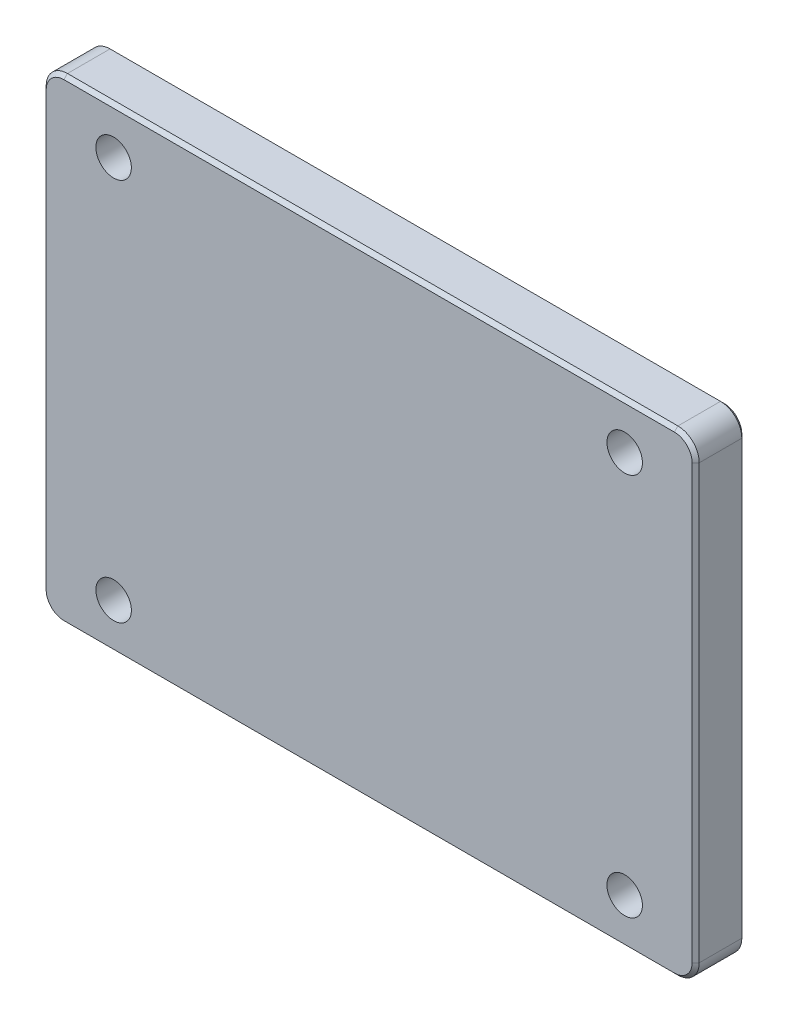
from build123d import *

# Parameters (mm, degrees)
SKETCH_1_W                  = 92
SKETCH_1_H                  = 67
EXTRUDE_1_DEPTH             = 7
FILLET_1_R                  = 3
SKETCH_2_R                  = 2.5
CUT_EXTRUDE_1_DEPTH         = 10
PATTERN_LINEAR_1_COUNT      = 2
PATTERN_LINEAR_1_PITCH      = 72
PATTERN_LINEAR_1_COUNT_DIR2 = 2
PATTERN_LINEAR_1_PITCH_DIR2 = 54
CHAMFER_1_SIZE              = 0.5


with BuildPart() as part:
    # 草图1 → 凸台-拉伸1 (new body)
    with BuildSketch(Plane.XY):
        Rectangle(SKETCH_1_W, SKETCH_1_H)
    extrude(amount=EXTRUDE_1_DEPTH)

    # 圆角1
    fillet_1_edges = [part.edges().sort_by_distance(p)[0] for p in [
        (46, -33.5, 3.5),
        (-46, -33.5, 3.5),
        (-46, 33.5, 3.5),
        (46, 33.5, 3.5),
    ]]
    fillet(fillet_1_edges, radius=FILLET_1_R)

    # 草图2 → 切除-拉伸1 (cut)
    with BuildSketch(Plane.XY.offset(7)):
        with Locations((-36, 27)):
            Circle(SKETCH_2_R)
    cut_extrude_1 = extrude(amount=-CUT_EXTRUDE_1_DEPTH, mode=Mode.SUBTRACT)

    # 阵列(线性)1: Cut-Extrude 1 2 × 2
    with Locations(*[(i * PATTERN_LINEAR_1_PITCH, -j * PATTERN_LINEAR_1_PITCH_DIR2, 0) for i in range(PATTERN_LINEAR_1_COUNT) for j in range(PATTERN_LINEAR_1_COUNT_DIR2) if (i, j) != (0, 0)]):
        add(cut_extrude_1, mode=Mode.SUBTRACT)

    # 倒角1
    chamfer_1_edges = [part.edges().sort_by_distance(p)[0] for p in [
        (46, 0, 0),
        (46, 0, 7),
        (0, -33.5, 0),
        (-46, 0, 0),
        (0, 33.5, 0),
        (-45.121320344, 32.621320344, 0),
        (45.121320344, 32.621320344, 0),
        (-45.121320344, -32.621320344, 0),
        (45.121320344, -32.621320344, 0),
        (0, -33.5, 7),
        (0, 33.5, 7),
        (-46, 0, 7),
        (-45.121320344, 32.621320344, 7),
        (45.121320344, 32.621320344, 7),
        (-45.121320344, -32.621320344, 7),
        (45.121320344, -32.621320344, 7),
    ]]
    chamfer(chamfer_1_edges, length=CHAMFER_1_SIZE)


solid = part.part
